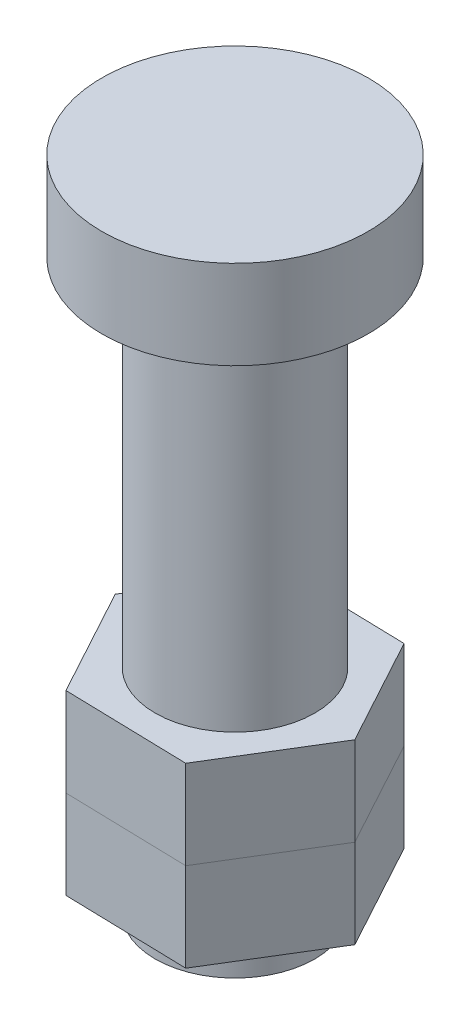
from build123d import *

# Parameters (mm, degrees)
SKETCH2_R           = 45
BOSS_EXTRUDE1_DEPTH = 50
LPATTERN1_COUNT     = 2
LPATTERN1_PITCH     = 50


with BuildPart() as part:
    # Sketch1 → Revolve1 (revolve)
    with BuildSketch(Plane.XY, mode=Mode.PRIVATE) as revolve1_sk:
        Polygon((0, 395.892857143), (75, 395.892857143), (75, 345.892857143), (45, 345.892857143), (45, 25.892857143), (0, 25.892857143), align=None)
    revolve(revolve1_sk.sketch.rotate(Axis((0, 0, 0), (0, 1, 0)), 90), axis=Axis((0, 0, 0), (0, 1, 0)))


with BuildPart() as body_2:
    # Sketch2 → Boss-Extrude1 (new body)
    with BuildSketch(Plane(origin=(0, 145.892857143, 0), x_dir=(-1, 0, 0), z_dir=(0, -1, 0))):
        Polygon((-33.101011459, -60.863150102), (36.158528413, -59.097891866), (69.259539873, 1.765258237), (33.101011459, 60.863150102), (-36.158528413, 59.097891866), (-69.259539873, -1.765258237), align=None)
        with Locations(Location((0, 0, 0), (0, 0, 90))):
            Circle(SKETCH2_R, mode=Mode.SUBTRACT)
    extrude(amount=BOSS_EXTRUDE1_DEPTH)


with BuildPart() as lpattern1_1:
    # LPattern1: pattern copy
    add(body_2.part.moved(Location(Vector(0, -1, 0) * (1 * LPATTERN1_PITCH))))


solid = Compound([part.part, body_2.part, lpattern1_1.part])
